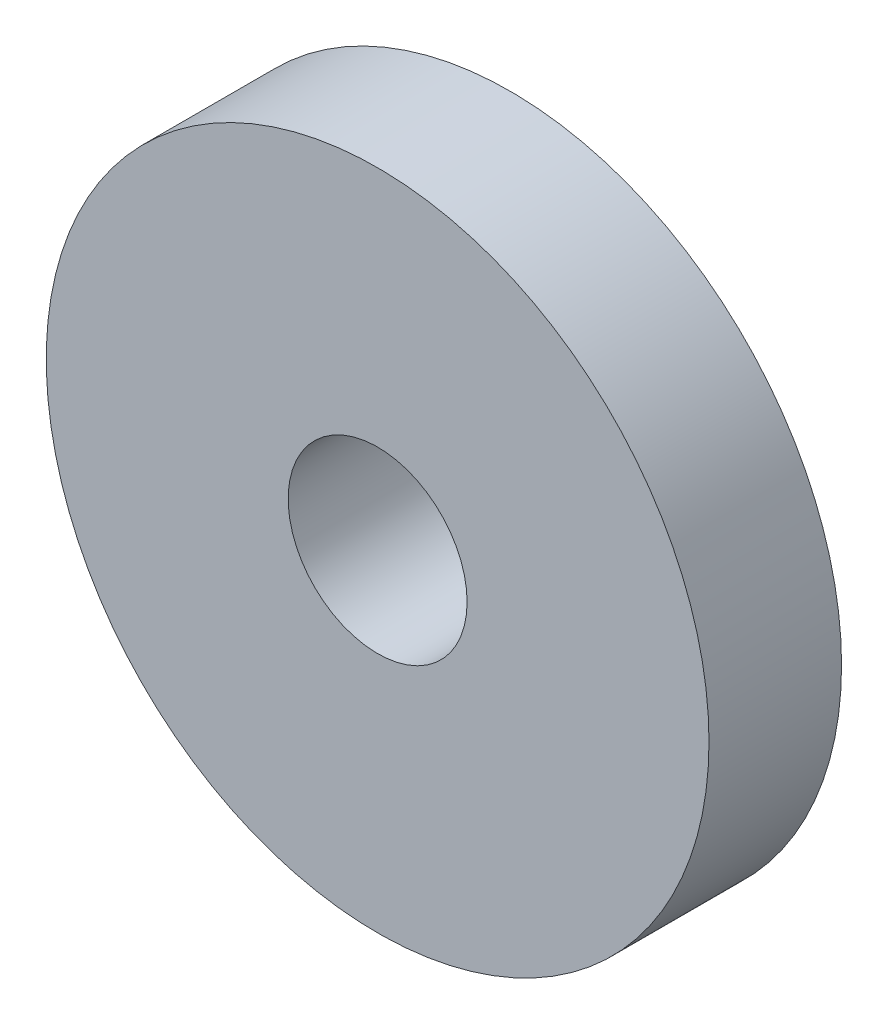
SolidWorks part; units mm, degrees
ref_plane "前视基准面" through (0, 0, 0) normal (0, 0, 1) x (1, 0, 0)
ref_plane "上视基准面" through (0, 0, 0) normal (0, 1, 0) x (1, 0, 0)
ref_plane "右视基准面" through (0, 0, 0) normal (1, 0, 0) x (0, 0, -1)
other "Configuration Table"
sketch "草图1" plane through (0, 0, 0) normal (0, 0, 1) x (1, 0, 0)
  circle A0 centre (0, 0) radius 30
  circle A1 centre (0, 0) radius 8.1
  point P0 (0, 0)
  dimension "D1" = 16.2
  dimension "D2" = 60
extrude "凸台-拉伸1" add sketch "草图1" against normal mid plane 12
